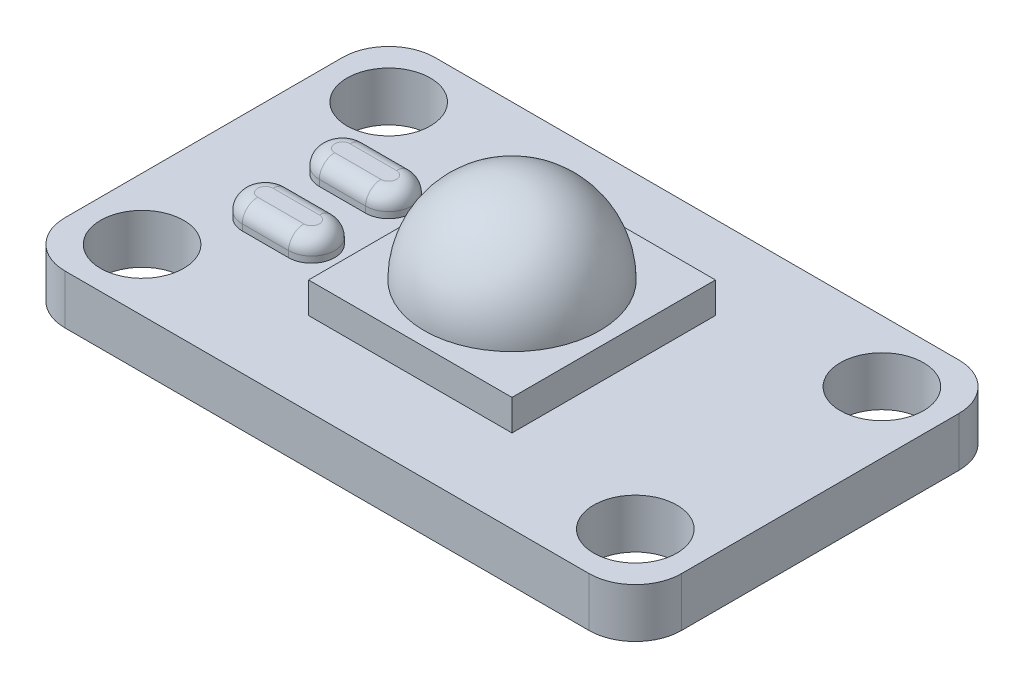
SolidWorks part; units mm, degrees
ref_plane "Front Plane" through (0, 0, 0) normal (0, 0, 1) x (1, 0, 0)
ref_plane "Top Plane" through (0, 0, 0) normal (0, 1, 0) x (1, 0, 0)
ref_plane "Right Plane" through (0, 0, 0) normal (1, 0, 0) x (0, 0, -1)
sketch "Aluminium base plate outline" plane through (0, 0, 0) normal (0, 1, 0) x (1, 0, 0)
  line L1 (-8.5, -6) -> (8.5, -6)
  line L2 (-10, -4.5) -> (-10, 4.5)
  line L3 (-8.5, 6) -> (8.5, 6)
  line L4 (10, -4.5) -> (10, 4.5)
  line L5 (-10, -6) -> (10, 6) construction
  line L6 (-10, 6) -> (10, -6) construction
  arc A0 (-8.5, -6) -> (-10, -4.5) centre (-8.5, -4.5) cw
  arc A1 (8.5, -6) -> (10, -4.5) centre (8.5, -4.5) ccw
  arc A2 (8.5, 6) -> (10, 4.5) centre (8.5, 4.5) cw
  arc A3 (-10, 4.5) -> (-8.5, 6) centre (-8.5, 4.5) cw
  point P0 (0, 0)
  dimension "D1" = 1.5
  dimension "D2" = 20
  dimension "D3" = 12
extrude "Aluminium base plate" add sketch "Aluminium base plate outline" along normal blind 1.6
sketch "Sketch7" plane through (0, 0, 0) normal (0, 1, 0) x (1, 0, 0)
  line L1 (-8, -4) -> (8, -4) construction
  line L2 (-8, -4) -> (-8, 4) construction
  line L3 (-8, 4) -> (8, 4) construction
  line L4 (8, -4) -> (8, 4) construction
  line L5 (-8, -4) -> (8, 4) construction
  line L6 (-8, 4) -> (8, -4) construction
  circle A0 centre (-8, -4) radius 1.35
  circle A1 centre (8, -4) radius 1.35
  circle A2 centre (8, 4) radius 1.35
  circle A3 centre (-8, 4) radius 1.35
  point P0 (0, 0)
  dimension "D3" = 2.7
  dimension "D1" = 8
  dimension "D2" = 16
extrude "Screw hole" cut sketch "Sketch7" along normal through all
sketch "？？？" plane through (0, 1.6, 0) normal (0, 1, 0) x (1, 0, 0)
  line L1 (-3.3, 3.3) -> (3.3, 3.3)
  line L2 (-3.3, 3.3) -> (-3.3, -3.3)
  line L3 (-3.3, -3.3) -> (3.3, -3.3)
  line L4 (3.3, 3.3) -> (3.3, -3.3)
  line L5 (-3.3, 3.3) -> (3.3, -3.3) construction
  line L6 (-3.3, -3.3) -> (3.3, 3.3) construction
  point P0 (0, 0)
  dimension "D1" = 6.6
extrude "LED bead board" add sketch "？？？" along normal blind 1 separate body
sketch "LED bead rotation base" plane through (0, 0, 0) normal (0, 0, 1) x (1, 0, 0)
  line L0 (0, 2.6) -> (2.85, 2.6)
  line L1 (0, 2.6) -> (0, 5.45)
  line L2 (-3.3, 2.6) -> (3.3, 2.6) construction
  arc A0 (0, 5.45) -> (2.85, 2.6) centre (0, 2.6) cw
  dimension "D1" = 2.85
revolve "LED bead" add sketch "LED bead rotation base" angle 360 about L1
sketch "Solder pad" plane through (0, 1.6, 0) normal (0, 1, 0) x (1, 0, 0)
  line L0 (-6.75, 1.25) -> (-5.25, 1.25) construction
  line L1 (-6.75, 2) -> (-5.25, 2)
  line L2 (-6.75, 0.5) -> (-5.25, 0.5)
  line L3 (-6.75, -1.25) -> (-5.25, -1.25) construction
  line L4 (-6.75, -0.5) -> (-5.25, -0.5)
  line L5 (-6.75, -2) -> (-5.25, -2)
  line L6 (-12.3939, 0) -> (49987.6061, 0) construction
  line L7 (-8.5, -6) -> (8.5, -6) construction
  line L8 (-10, 4.5) -> (-10, -4.5) construction
  arc A0 (-6.75, 2) -> (-6.75, 0.5) centre (-6.75, 1.25) ccw
  arc A1 (-5.25, 0.5) -> (-5.25, 2) centre (-5.25, 1.25) ccw
  arc A2 (-6.75, -0.5) -> (-6.75, -2) centre (-6.75, -1.25) ccw
  arc A3 (-5.25, -2) -> (-5.25, -0.5) centre (-5.25, -1.25) ccw
  point P2 (-6, 1.25)
  point P7 (-6, -1.25)
  dimension "D1" = 0.75
  dimension "D2" = 1.5
  dimension "D3" = 4.75
  dimension "D4" = 4
extrude "Solder joint base outline" add sketch "Solder pad" along normal blind 0.7 separate body
fillet "Solder joint 1" radius 0.5 4 edges at (-6, 2.3, -2) (-4.5, 2.3, -1.25) (-6, 2.3, -0.5) (-7.5, 2.3, -1.25)
fillet "Solder joint 2" radius 0.5 4 edges at (-6, 2.3, 2) (-7.5, 2.3, 1.25) (-6, 2.3, 0.5) (-4.5, 2.3, 1.25)
